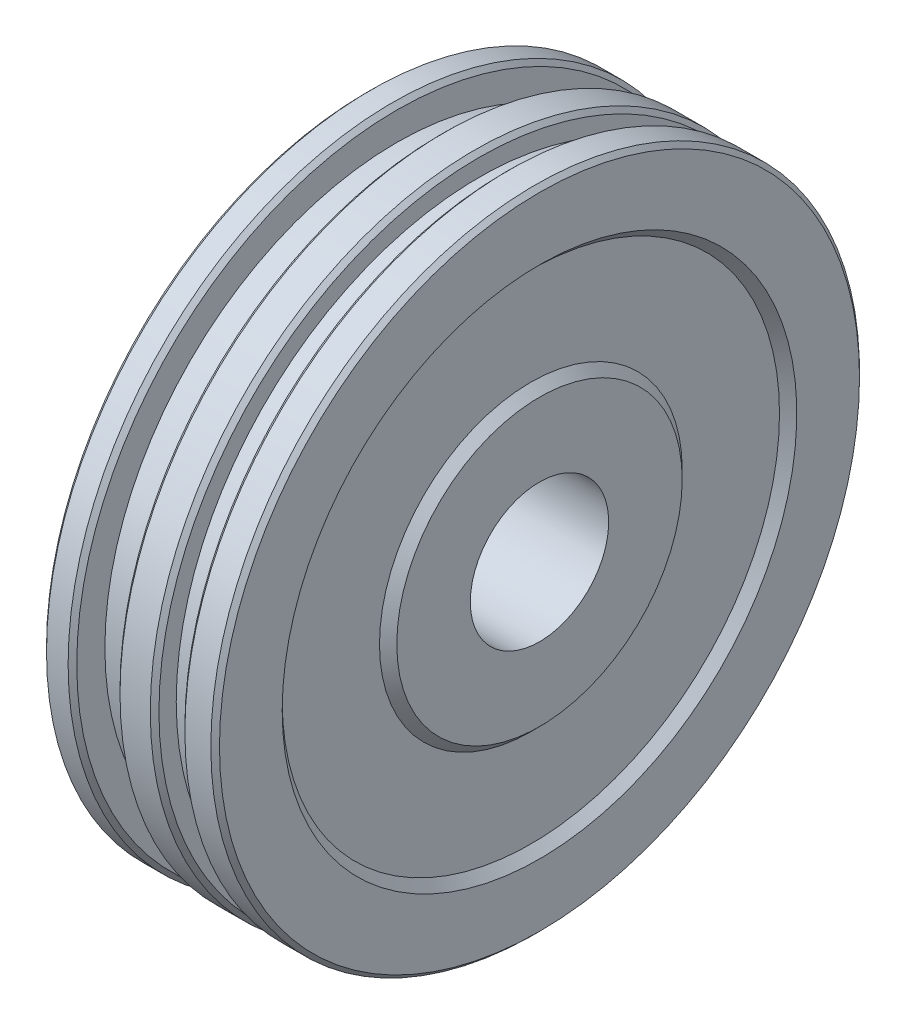
from build123d import *

# Parameters (mm, degrees)
CHAMFER_1_SIZE = 1


with BuildPart() as part:
    # 草图1 → 旋转1 (revolve)
    with BuildSketch(Plane.XY, mode=Mode.PRIVATE) as revolve_1_sk:
        Polygon((0, 51), (0, 75), (7, 75), (7, 67.5), (17, 67.5), (17, 75), (26, 75), (26, 70), (32, 70), (32, 75), (40, 75), (40, 59.5), (38, 57.5), (38, 35), (40, 33), (40, 16), (13, 16), (13, 51), align=None)
    revolve(revolve_1_sk.sketch.rotate(Axis((0, 0, 0), (1, 0, 0)), 90), axis=Axis((0, 0, 0), (1, 0, 0)))

    # 倒角1
    chamfer_1_edges = [part.edges().sort_by_distance(p)[0] for p in [
        (40, 0, -75),
        (32, 0, -75),
        (26, 0, -75),
        (17, 0, -75),
        (7, 0, -75),
        (0, 0, -75),
    ]]
    chamfer(chamfer_1_edges, length=CHAMFER_1_SIZE)


solid = part.part
